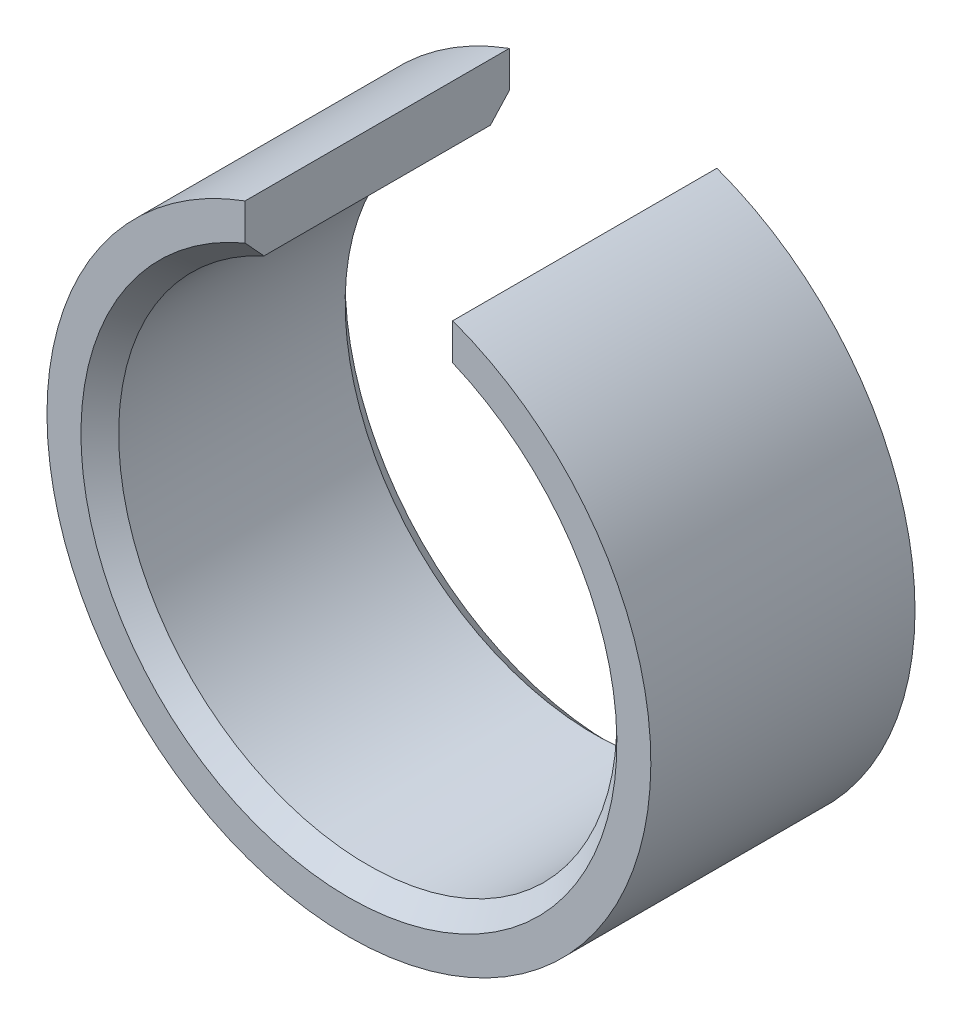
SolidWorks part; units mm, degrees
material "6061-T6 (GB)"
ref_plane "Front Plane" through (0, 0, 0) normal (0, 0, 1) x (1, 0, 0)
ref_plane "Top Plane" through (0, 0, 0) normal (0, 1, 0) x (1, 0, 0)
ref_plane "Right Plane" through (0, 0, 0) normal (1, 0, 0) x (0, 0, -1)
sketch "Sketch1" plane through (0, 0, 0) normal (0, 0, 1) x (1, 0, 0)
  circle A0 centre (0, 0) radius 6.6
  circle A1 centre (0, 0) radius 8
  dimension "D1" = 13.2
  dimension "D2" = 16
extrude "Boss-Extrude1" add sketch "Sketch1" along normal blind 7
sketch "Sketch2" plane through (0, 0, 7) normal (0, 0, 1) x (1, 0, 0)
  line L0 (0, 0) -> (0, 6.6) construction
  line L1 (2.75, 3.8711) -> (-2.75, 3.8711)
  line L2 (2.75, 3.8711) -> (2.75, 11.0375)
  line L3 (2.75, 11.0375) -> (-2.75, 11.0375)
  line L4 (-2.75, 3.8711) -> (-2.75, 11.0375)
  line L5 (2.75, 3.8711) -> (-2.75, 11.0375) construction
  line L6 (2.75, 11.0375) -> (-2.75, 3.8711) construction
  circle A0 centre (0, 0) radius 6.6 construction
  point P0 (0, 7.4543)
  dimension "D1" = 5.5
extrude "Cut-Extrude1" cut sketch "Sketch2" against normal through all
chamfer "Chamfer1" distance 0.5 angle 45 2 edges at (0, -6.6, 0) (0, -6.6, 7)
